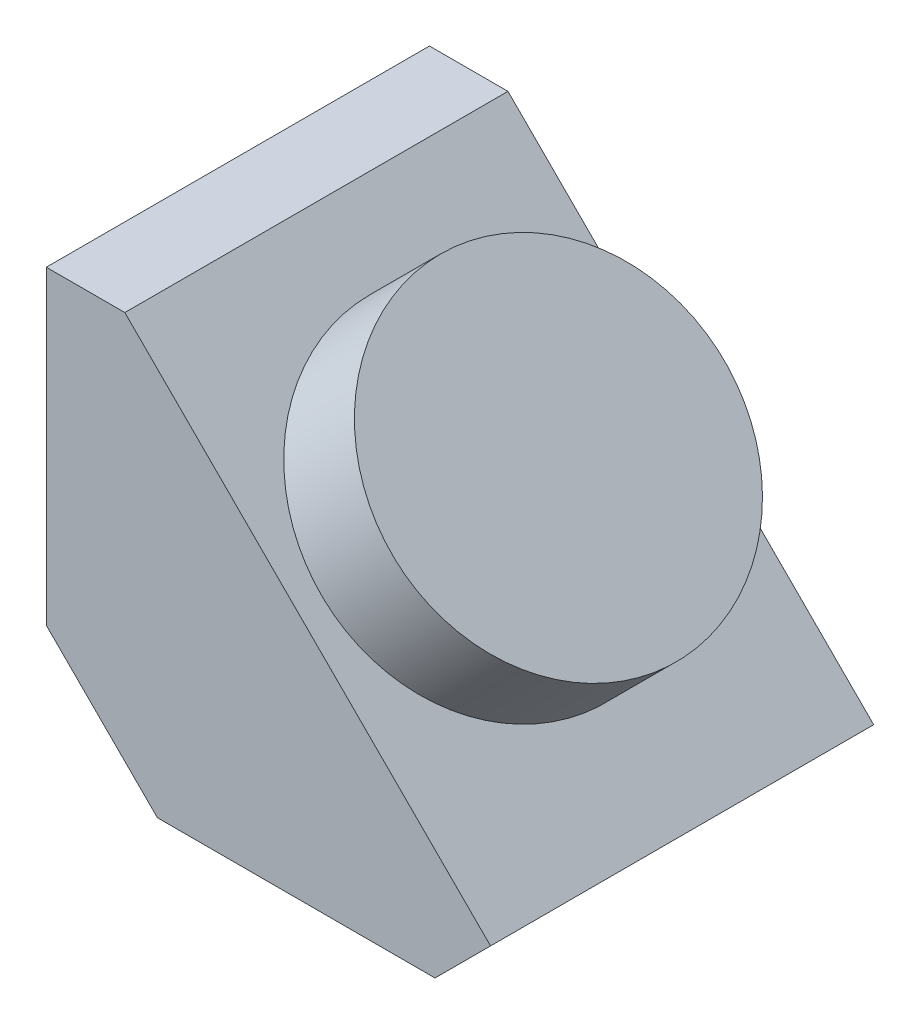
from build123d import *
from OCP.BRepFilletAPI import BRepFilletAPI_MakeChamfer

# Parameters (mm, degrees)
EXTRUDE_1_DEPTH = 69
CHAMFER_1_SIZE  = 20
SKETCH_3_R      = 30
EXTRUDE_2_DEPTH = 18
CHAMFER_2_SIZE  = 20
CHAMFER_2_SIZE2 = 14.142135624


with BuildPart() as part:
    # 草图1 → 凸台-拉伸1 (new body)
    with BuildSketch(Plane.XY):
        Polygon((0, 0), (0, -90), (90, -90), align=None)
    extrude(amount=EXTRUDE_1_DEPTH)

    # 倒角1
    chamfer_1_edges = [part.edges().sort_by_distance(p)[0] for p in [
        (0, -90, 34.5),
    ]]
    chamfer(chamfer_1_edges, length=CHAMFER_1_SIZE)

    # 草图3 → 凸台-拉伸2 (add)
    with BuildSketch(Plane(origin=(0, 0, 0), x_dir=(0, 0, -1), z_dir=(0.7071067811865475, 0.7071067811865476, 0))):
        with Locations(Location((-34.5, -63.639610307, 0), (0, 0, 90))):
            Circle(SKETCH_3_R)
    extrude(amount=EXTRUDE_2_DEPTH)

    # 倒角2: one chamfer whose edges measure the first distance from different faces: ONE call of the kernel's chamfer builder (chamfer() names one face for all edges)
    chamfer_2_edges_1 = [part.edges().sort_by_distance(p)[0] for p in [
        (90, -90, 34.5),
    ]]
    chamfer_2_side_1 = [part.faces().sort_by_distance(p)[0] for p in [
        (55, -90, 34.5),
    ]]
    chamfer_2_edges_2 = [part.edges().sort_by_distance(p)[0] for p in [
        (0, 0, 34.5),
    ]]
    chamfer_2_side_2 = [part.faces().sort_by_distance(p)[0] for p in [
        (88.976256868, -88.976256868, 34.5),
    ]]
    chamfer_2 = BRepFilletAPI_MakeChamfer(part.part.solid().wrapped)
    for e in chamfer_2_edges_1:
        chamfer_2.Add(CHAMFER_2_SIZE, CHAMFER_2_SIZE2, e.wrapped, chamfer_2_side_1[0].wrapped)  # the first distance lies on this face
    for e in chamfer_2_edges_2:
        chamfer_2.Add(CHAMFER_2_SIZE, CHAMFER_2_SIZE2, e.wrapped, chamfer_2_side_2[0].wrapped)  # the first distance lies on this face
    add(Compound.cast(chamfer_2.Shape()), mode=Mode.REPLACE)


solid = part.part
